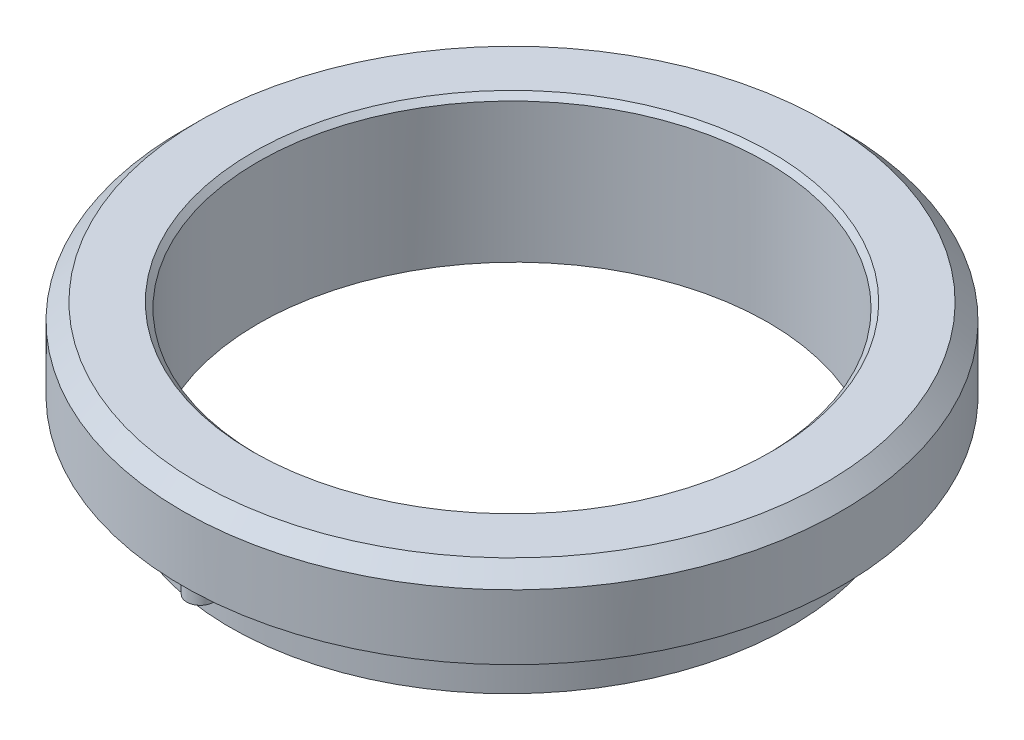
SolidWorks part; units mm, degrees
material "6061-T6 (SS)"
ref_plane "前视基准面" through (0, 0, 0) normal (0, 0, 1) x (1, 0, 0)
ref_plane "上视基准面" through (0, 0, 0) normal (0, 1, 0) x (1, 0, 0)
ref_plane "右视基准面" through (0, 0, 0) normal (1, 0, 0) x (0, 0, -1)
sketch "草图1" plane through (0, 0, 0) normal (0, 0, 1) x (1, 0, 0)
  line L0 (23.5, -7.5) -> (23.5, 7.5)
  line L4 (30.5, 7.5) -> (30.5, 0)
  line L5 (30.5, 0) -> (27.35, 0)
  line L6 (25.85, 1) -> (25.85, -7.5)
  line L8 (0, 0) -> (0, 20.5777) construction
  line L9 (55, 0) -> (-55, 0) construction
  line L13 (25.85, -7.5) -> (23.5, -7.5)
  line L15 (30.5, 7.5) -> (23.5, 7.5)
  line L16 (27.35, 0) -> (27.35, 1)
  line L17 (27.35, 1) -> (25.85, 1)
  dimension "D1" = 1.5
  dimension "D2" = 15
  dimension "D3" = 7.5
  dimension "D4" = 47
  dimension "D5" = 51.7
  dimension "D6" = 1
  dimension "D7" = 61
revolve "旋转1" add sketch "草图1" angle 360 about L8
sketch "草图2" plane through (0, 0, 0) normal (0, 0, 1) x (1, 0, 0)
  line L0 (-25.85, -6) -> (25.85, -5.5488)
  line L1 (-25.85, 1) -> (-25.85, -7.5) construction
  line L3 (25.85, -5.5488) -> (25.85, -7.5)
  line L4 (25.85, -7.5) -> (-25.85, -7.5)
  line L5 (-25.85, -7.5) -> (-25.85, -6)
  line L9 (-30.5, 0) -> (30.5, 0) construction
  dimension "D1" = 0.5
  dimension "D2" = 5.5488
  dimension "D3" = 6
extrude "切除-拉伸1" cut sketch "草图2" against normal through all both and the other way through all
chamfer "倒角1" distance 0.5 angle 45 1 edges at (0, 7.5, -23.5)
chamfer "倒角2" distance 1.5 angle 45 1 edges at (0, 7.5, -30.5)
sketch "草图3" plane through (0, 0, 0) normal (0, -1, 0) x (1, 0, 0)
  circle A0 centre (0, 28.85) radius 1.25
  dimension "D1" = 2.5
  dimension "D2" = 28.85
extrude "凸台-拉伸1" add sketch "草图3" along normal blind 1.5
